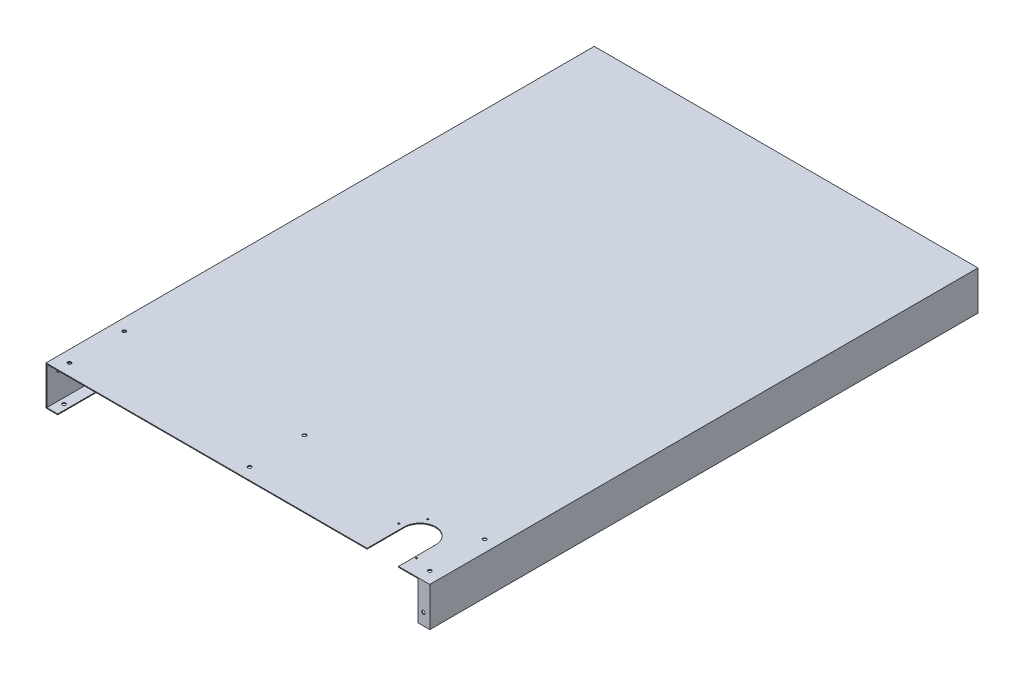
SolidWorks part; units mm, degrees
ref_plane "前视" through (0, 0, 0) normal (0, 0, 1) x (1, 0, 0)
ref_plane "上视" through (0, 0, 0) normal (0, 1, 0) x (1, 0, 0)
ref_plane "右视" through (0, 0, 0) normal (1, 0, 0) x (0, 0, -1)
sketch "草图1" plane through (0, 0, 0) normal (0, 1, 0) x (1, 0, 0)
  line L0 (0, 0) -> (0, 34.4083) construction
  line L1 (-490, 700) -> (490, 700)
  line L2 (-490, 700) -> (-490, -700)
  line L3 (-490, -700) -> (490, -700)
  line L4 (490, 700) -> (490, -700)
  line L5 (0, 0) -> (51.7131, 0) construction
  dimension "D1" = 1400
  dimension "D2" = 980
  dimension "D3" = 700
  dimension "D4" = 490
extrude "凸台-拉伸1" add sketch "草图1" against normal blind 100
shell "抽壳1" thickness 2
sketch "草图3" plane through (0, 0, 0) normal (0, 1, 0) x (1, 0, 0)
  line L0 (-490, -700) -> (490, -700) construction
  line L1 (330, -700) -> (410, -700)
  line L2 (330, -700) -> (330, -604.5)
  line L3 (490, -700) -> (490, 700) construction
  line L4 (410, -700) -> (410, -604.5)
  line L5 (370, -700) -> (370, -512.3898) construction
  arc A0 (410, -604.5) -> (330, -604.5) centre (370, -605) ccw
  dimension "D4" = 40.0031
  dimension "D1" = 95
  dimension "D3" = 80
  dimension "D5" = 80
extrude "切除-拉伸1" cut sketch "草图3" against normal blind 20
sketch "草图5" plane through (0, 0, 700) normal (0, 0, 1) x (1, 0, 0)
  line L1 (-488, -2) -> (488, -2)
  line L2 (-488, -2) -> (-488, -100)
  line L3 (-488, -100) -> (488, -100)
  line L4 (488, -2) -> (488, -100)
extrude "切除-拉伸2" cut sketch "草图5" against normal blind 20
sketch "草图6" plane through (0, -100, 0) normal (0, -1, 0) x (1, 0, 0)
  line L0 (490, 700) -> (490, -700)
  line L1 (490, -700) -> (-490, -700)
  line L2 (-490, -700) -> (-490, 700)
  line L3 (-490, 700) -> (-460, 700)
  line L4 (330, 700) -> (-488, 700) construction
  line L5 (490, 700) -> (460, 700)
  line L7 (488, 700) -> (410, 700) construction
  line L8 (460, 700) -> (460, -670)
  line L9 (-460, 700) -> (-460, -670)
  line L10 (-460, -670) -> (460, -670)
  dimension "D1" = 30
  dimension "D2" = 30
  dimension "D3" = 30
extrude "凸台-拉伸2" add sketch "草图6" against normal blind 2
sketch "草图7" plane through (488, 0, 0) normal (-1, 0, 0) x (0, 0, 1)
  line L0 (700, -98) -> (-698, -98) construction
  line L1 (700, -2) -> (698, -2)
  line L2 (700, -2) -> (700, -98)
  line L3 (700, -98) -> (698, -98)
  line L4 (698, -2) -> (698, -98)
  dimension "D1" = 2
extrude "凸台-拉伸3" add sketch "草图7" along normal blind 28
sketch "草图8" plane through (0, -100, 0) normal (0, -1, 0) x (1, 0, 0)
  line L0 (490, 0) -> (-730.4351, 0) construction
  line L1 (490, 700) -> (490, -700) construction
  line L16 (0, -684) -> (0, 1226.0983) construction
  line L17 (-490, 700) -> (-460, 700) construction
  line L19 (474, 700) -> (474, -684)
  line L20 (474, -684) -> (-474, -684)
  line L21 (-474, -684) -> (-474, 700)
  line L22 (474, 700) -> (474, -684) construction
  line L23 (474, -684) -> (-474, -684) construction
  line L24 (-474, -684) -> (-474, 700) construction
  circle A1 centre (-474, 670) radius 4.5
  circle A2 centre (-474, 0) radius 4.5
  circle A3 centre (-474, -684) radius 4.5
  circle A4 centre (0, -684) radius 4.5
  circle A5 centre (474, -684) radius 4.5
  circle A6 centre (474, 0) radius 4.5
  circle A7 centre (474, 670) radius 4.5
  dimension "D2" = 9
  dimension "D3" = 9
  dimension "D4" = 9
  dimension "D5" = 9
  dimension "D6" = 30
  dimension "D1" = 14
extrude "切除-拉伸3" cut sketch "草图8" against normal blind 10
sketch "草图9" plane through (0, 0, 698) normal (0, 0, -1) x (-1, 0, 0)
  line L0 (-474, -98) -> (-474, 38.699) construction
  line L1 (-460, -98) -> (-488, -98) construction
  line L2 (-460, -100) -> (-490, -100) construction
  circle A0 centre (-474, -70) radius 4.5
  dimension "D1" = 9
  dimension "D2" = 30
extrude "切除-拉伸4" cut sketch "草图9" against normal blind 10
sketch "草图10" plane through (-488, 0, 0) normal (1, 0, 0) x (0, 0, -1)
  line L1 (-700, -2) -> (-700, -98) construction
  line L2 (-700, 0) -> (700, 0) construction
  line L3 (698, -30) -> (-700, -30) construction
  circle A0 centre (-670, -30) radius 4.5
  circle A1 centre (-330, -30) radius 4.5
  dimension "D2" = 9
  dimension "D3" = 9
  dimension "D4" = 30
  dimension "D5" = 340
  dimension "D1" = 30
extrude "切除-拉伸5" cut sketch "草图10" against normal blind 10
sketch "草图11" plane through (0, 0, 0) normal (0, 1, 0) x (1, 0, 0)
  line L2 (-460, 700) -> (-460, -700)
  line L3 (-460, 700) -> (-460, -700) construction
  line L4 (0, 700) -> (0, -875.333) construction
  line L5 (460, -700) -> (460, 700)
  line L6 (460, -700) -> (460, 700) construction
  line L7 (490, 700) -> (-490, 700) construction
  line L8 (-689.2719, -530) -> (794.9885, -530) construction
  line L9 (-490, -700) -> (330, -700) construction
  circle A0 centre (-460, -670) radius 4.5
  circle A1 centre (0, -530) radius 4.5
  circle A2 centre (460, -530) radius 4.5
  circle A3 centre (-460, -530) radius 4.5
  circle A4 centre (0, -670) radius 4.5
  circle A5 centre (460, -670) radius 4.5
  dimension "D3" = 9
  dimension "D4" = 9
  dimension "D5" = 9
  dimension "D6" = 9
  dimension "D7" = 30
  dimension "D8" = 30
  dimension "D9" = 140
  dimension "D1" = 30
  dimension "D2" = 30
extrude "切除-拉伸6" cut sketch "草图11" against normal blind 10
hole_wizard "M5 螺纹孔1" positions "草图13" profile "草图12" tap size "M5" standard "GB"
sketch "草图13" plane through (0, 0, 0) normal (0, 1, 0) x (-1, 0, 0)
  line L0 (-370, 659) -> (-505.0082, 659) construction
  line L2 (-343, 558.2346) -> (-370, 605) construction
  line L3 (-370, 605) -> (-370, 514.1532) construction
  circle A0 centre (-370, 605) radius 54 construction
  point P0 (-343, 558.2346)
  point P1 (-316, 605)
  point P3 (-415, 659)
  dimension "D1" = 108
  dimension "D2" = 45
  dimension "D3" = 30
sketch "草图12" plane through (343, 0, 558.2346) normal (1, 0, 0) x (0, 0, 1)
  line L0 (0, 0) -> (0, 1261.2618)
  line L1 (0, 1261.2618) -> (2.1, 1260)
  line L2 (2.1, 1260) -> (2.1, 0)
  line L5 (2.1, 0) -> (0, 0)
  line L10 (0, 1261.2618) -> (-2.1, 1260) construction
  line L11 (0, -6.35) -> (0, 107.95) construction
  dimension "螺纹孔钻头直径" = 4.2
  dimension "螺纹孔钻头深度" = 1260
  dimension "导头角度" = 118
cosmetic thread "孔螺蚊线1" parameters "D1"=2, "D2"=5
cosmetic thread "孔螺蚊线2" parameters "D1"=2, "D2"=5
cosmetic thread "孔螺蚊线3" parameters "D1"=2, "D2"=5
